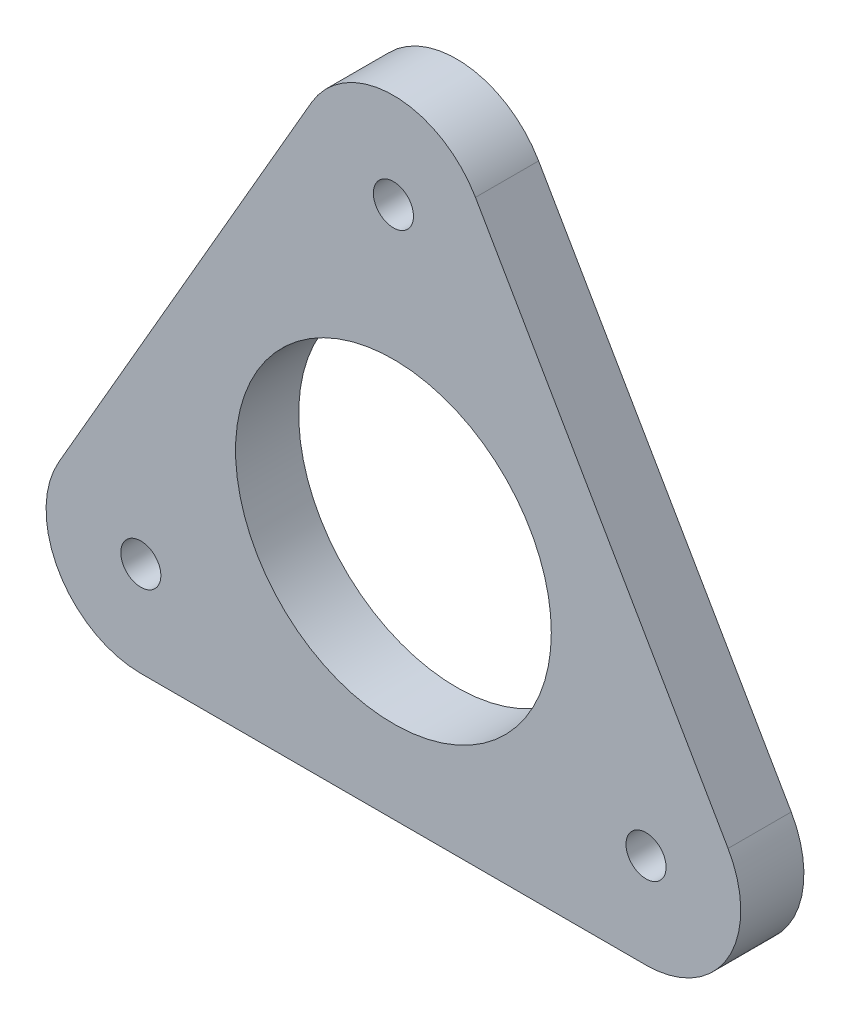
SolidWorks part; units mm, degrees
ref_plane "Front Plane" through (0, 0, 0) normal (0, 0, 1) x (1, 0, 0)
ref_plane "Top Plane" through (0, 0, 0) normal (0, 1, 0) x (1, 0, 0)
ref_plane "Right Plane" through (0, 0, 0) normal (1, 0, 0) x (0, 0, -1)
sketch "Sketch1" plane through (0, 0, 0) normal (0, 0, 1) x (1, 0, 0)
  line L0 (-52.9904, -15.594) -> (-12.9904, 53.688)
  line L1 (0, 46.188) -> (-40, -23.094) construction
  line L2 (-40, -23.094) -> (40, -23.094) construction
  line L3 (40, -23.094) -> (0, 46.188) construction
  line L4 (12.9904, 53.688) -> (52.9904, -15.594)
  line L5 (-40, -38.094) -> (40, -38.094)
  circle A0 centre (0, 0) radius 23.094 construction
  arc A1 (-52.9904, -15.594) -> (-40, -38.094) centre (-40, -23.094) ccw
  arc A2 (40, -38.094) -> (52.9904, -15.594) centre (40, -23.094) ccw
  arc A3 (12.9904, 53.688) -> (-12.9904, 53.688) centre (0, 46.188) ccw
  circle A4 centre (-40, -23.094) radius 3.175
  circle A5 centre (40, -23.094) radius 3.175
  circle A6 centre (0, 46.188) radius 3.175
  circle A7 centre (0, 0) radius 25
  dimension "D2" = 30
  dimension "D3" = 6.35
  dimension "D4" = 50
  dimension "D1" = 80
extrude "Boss-Extrude1" add sketch "Sketch1" along normal blind 10
sketch "Sketch2" plane through (0, 0, 0) normal (0, 0, 1) x (1, 0, 0)
  line L0 (-40, -23.094) -> (0, 0) construction
  line L1 (-39.6817, -27.5827) -> (-46.8575, -28.0915)
  line L2 (-43.7282, -20.574) -> (-47.7567, -26.534)
  line L3 (-4.0465, 48.1568) -> (-0.8992, 54.6255)
  line L4 (4.0465, 48.1568) -> (0.8992, 54.6255)
  line L5 (43.7282, -20.574) -> (47.7567, -26.534)
  line L6 (39.6817, -27.5827) -> (46.8575, -28.0915)
  line L7 (52.9904, -30.594) -> (0, 0) construction
  arc A0 (-39.6817, -27.5827) -> (-43.7282, -20.574) centre (-40, -23.094) ccw
  circle A1 centre (-40, -23.094) radius 3.175
  arc A2 (-47.7567, -26.534) -> (-46.8575, -28.0915) centre (-46.9282, -27.094) ccw
  arc A3 (-4.0465, 48.1568) -> (4.0465, 48.1568) centre (0, 46.188) ccw
  circle A4 centre (0, 46.188) radius 3.175
  arc A5 (0.8992, 54.6255) -> (-0.8992, 54.6255) centre (0, 54.188) ccw
  arc A6 (43.7282, -20.574) -> (39.6817, -27.5827) centre (40, -23.094) ccw
  circle A7 centre (40, -23.094) radius 3.175
  arc A8 (46.8575, -28.0915) -> (47.7567, -26.534) centre (46.9282, -27.094) ccw
  arc A9 (40, -38.094) -> (52.9904, -15.594) centre (40, -23.094) ccw construction
  point P26 (0, 0)
  point P28 (0, 0)
  dimension "D1" = 9
  dimension "D2" = 2
  dimension "D3" = 8
  dimension "D4" = 3
extrude "Cut-Extrude1" cut sketch "Sketch2" along normal blind 3
scale "Scale ratio 1" scale about origin uniform scaling yes scale factor 1.3
